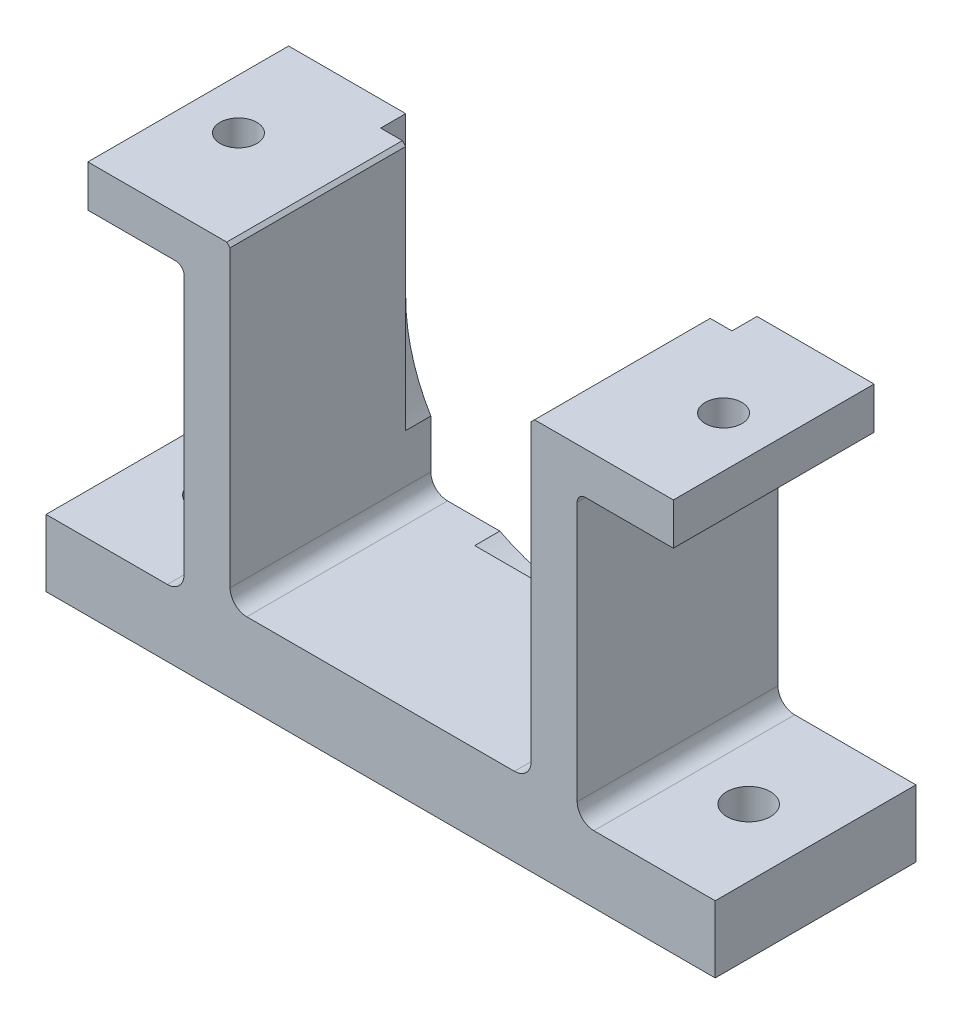
SolidWorks part; units mm, degrees
ref_plane "Front Plane" through (0, 0, 0) normal (0, 0, 1) x (1, 0, 0)
ref_plane "Top Plane" through (0, 0, 0) normal (0, 1, 0) x (1, 0, 0)
ref_plane "Right Plane" through (0, 0, 0) normal (1, 0, 0) x (0, 0, -1)
sketch "Sketch1" plane through (0, 0, 0) normal (0, 0, 1) x (1, 0, 0)
  line L0 (0, 0) -> (0, 168.5075) construction
  line L1 (-200, 0) -> (200, 0)
  line L2 (-200, 0) -> (-200, 40)
  line L3 (-200, 40) -> (-127.5, 40)
  line L4 (-117.5, 50) -> (-117.5, 205)
  line L5 (-122.5, 210) -> (-175, 210)
  line L6 (-175, 210) -> (-175, 235)
  line L7 (-175, 235) -> (-92, 235)
  line L8 (-90, 233) -> (-90, 57)
  line L9 (-80, 47) -> (80, 47)
  line L10 (200, 0) -> (200, 40)
  line L11 (175, 210) -> (175, 235)
  line L12 (90, 233) -> (90, 57)
  line L13 (175, 235) -> (92, 235)
  line L14 (122.5, 210) -> (175, 210)
  line L15 (117.5, 50) -> (117.5, 205)
  line L16 (200, 40) -> (127.5, 40)
  line L17 (-92, 235) -> (-90, 233)
  line L18 (92, 235) -> (90, 233)
  arc A0 (127.5, 40) -> (117.5, 50) centre (127.5, 50) cw
  arc A1 (-117.5, 50) -> (-127.5, 40) centre (-127.5, 50) cw
  arc A2 (80, 47) -> (90, 57) centre (80, 57) ccw
  arc A3 (-80, 47) -> (-90, 57) centre (-80, 57) cw
  arc A4 (122.5, 210) -> (117.5, 205) centre (122.5, 205) ccw
  arc A5 (-117.5, 205) -> (-122.5, 210) centre (-122.5, 205) ccw
  point P6 (0, 0)
  point P12 (-90, 235)
  point P14 (90, 235)
  point P18 (0, 47)
  point P23 (117.5, 40)
  point P26 (-117.5, 40)
  point P29 (90, 47)
  point P32 (-90, 47)
  point P35 (117.5, 210)
  point P38 (-117.5, 210)
  dimension "D9" = 10
  dimension "D10" = 5
  dimension "D1" = 400
  dimension "D2" = 40
  dimension "D3" = 25
  dimension "D4" = 235
  dimension "D5" = 350
  dimension "D6" = 235
  dimension "D7" = 180
  dimension "D8" = 188
extrude "Boss-Extrude1" add sketch "Sketch1" along normal mid plane 120
sketch "Sketch2" plane through (0, 0, 0) normal (0, -1, 0) x (1, 0, 0)
  line L0 (-200, 0) -> (200, 0) construction
  line L1 (-200, 60) -> (-200, -60) construction
  line L2 (200, 60) -> (200, -60) construction
  line L3 (0, 0) -> (0, 111.7564) construction
  circle A0 centre (-160, 0) radius 13
  circle A1 centre (160, 0) radius 13
  dimension "D1" = 26
  dimension "D2" = 320
extrude "Cut-Extrude1" cut sketch "Sketch2" against normal blind 87
sketch "Sketch3" plane through (0, 235, 0) normal (0, 1, 0) x (1, 0, 0)
  line L0 (-175, 0) -> (64.4267, 0) construction
  line L1 (-175, -60) -> (-175, 60) construction
  line L2 (0, 0) -> (0, 92.9914) construction
  circle A0 centre (-145, 0) radius 11
  circle A1 centre (145, 0) radius 11
  dimension "D1" = 22
  dimension "D2" = 290
extrude "Cut-Extrude2" cut sketch "Sketch3" against normal blind 87
sketch "Sketch4" plane through (0, 0, -60) normal (0, 0, -1) x (-1, 0, 0)
  line L0 (-105, 140) -> (-105, 340)
  line L1 (-105, 340) -> (105, 340)
  line L2 (105, 340) -> (105, 140)
  arc A0 (-105, 140) -> (105, 140) centre (0, 140) ccw
  dimension "D1" = 210
  dimension "D2" = 140
  dimension "D3" = 200
extrude "Cut-Extrude3" cut sketch "Sketch4" against normal blind 15
